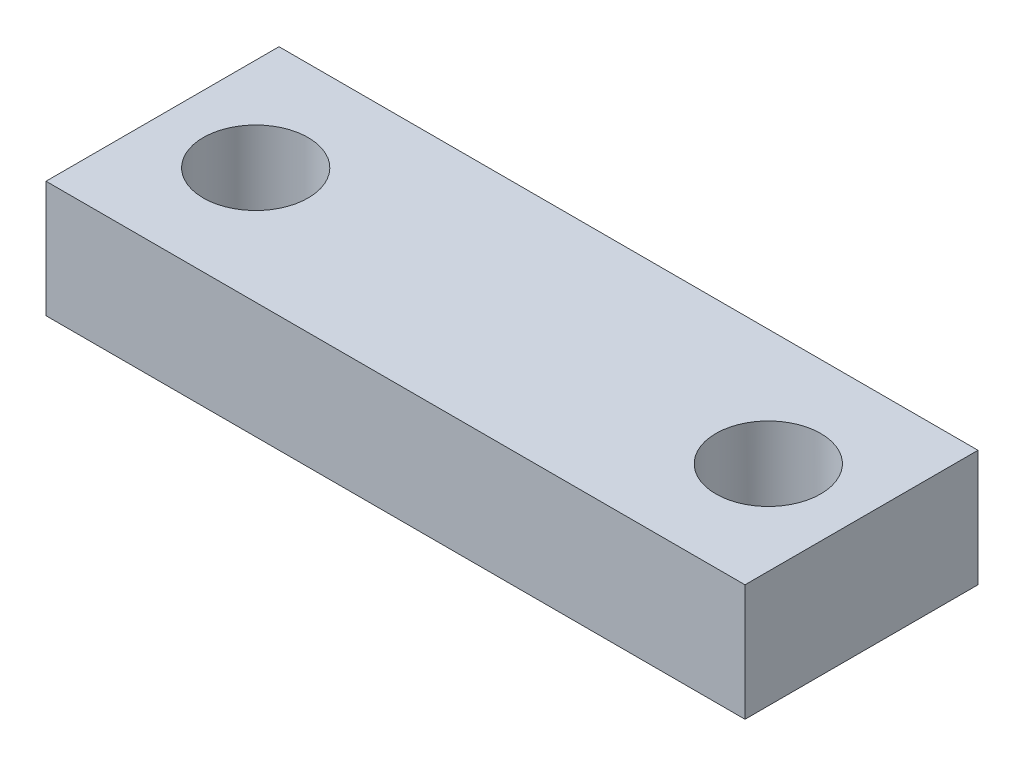
from build123d import *

# Parameters (mm, degrees)
SKETCH1_W           = 30
SKETCH1_H           = 10
BOSS_EXTRUDE1_DEPTH = 5
SKETCH2_R           = 2.25
CUT_EXTRUDE1_DEPTH  = 10


with BuildPart() as part:
    # Sketch1 → Boss-Extrude1 (new body)
    with BuildSketch(Plane(origin=(0, 0, 0), x_dir=(1, 0, 0), z_dir=(0, 1, 0))):
        Rectangle(SKETCH1_W, SKETCH1_H)
    extrude(amount=BOSS_EXTRUDE1_DEPTH)

    # Sketch2 → Cut-Extrude1 (cut)
    with BuildSketch(Plane(origin=(0, 5, 0), x_dir=(1, 0, 0), z_dir=(0, 1, 0))):
        with Locations(Location((-11, 0, 0), (0, 0, 270))):
            Circle(SKETCH2_R)
        with Locations(Location((11, 0, 0), (0, 0, 270))):
            Circle(SKETCH2_R)
    extrude(amount=-CUT_EXTRUDE1_DEPTH, mode=Mode.SUBTRACT)


solid = part.part
